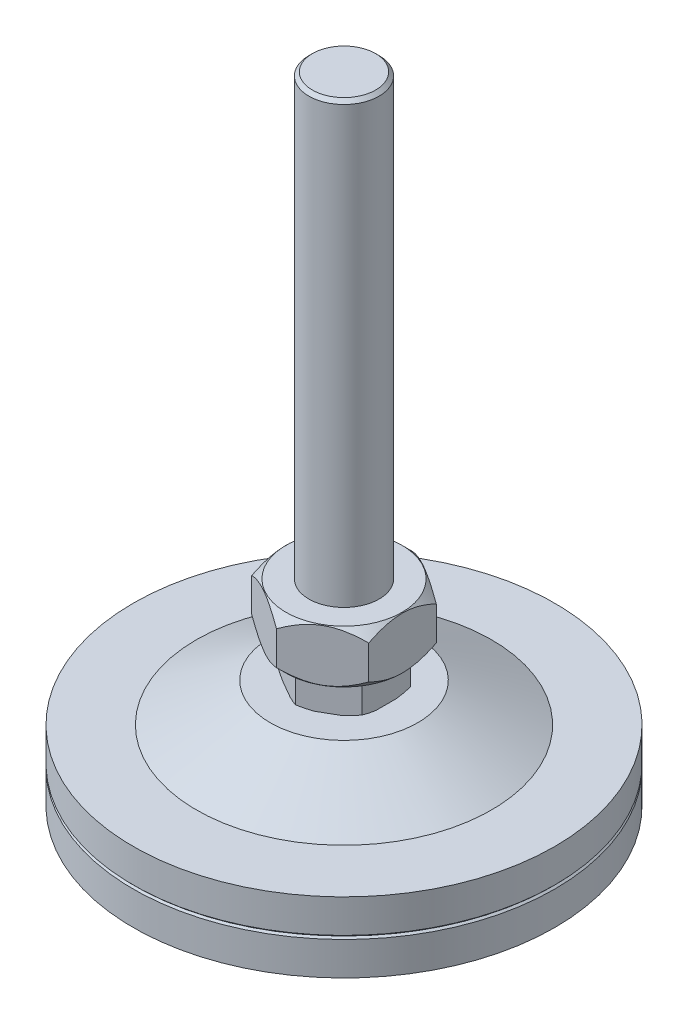
from build123d import *

# Parameters (mm, degrees)
BOSS_EXTRUDE1_DEPTH = 9
BOSS_EXTRUDE2_START = 15
SKETCH5_R           = 10
BOSS_EXTRUDE2_DEPTH = 15
CHAMFER1_SIZE       = 1


with BuildPart() as part:
    # Sketch1 → Revolve1 (revolve)
    with BuildSketch(Plane.XY, mode=Mode.PRIVATE) as revolve1_sk:
        Polygon((35, 0), (60, 0), (60, 9.5), (59.5, 10), (60, 10.5), (60, 20), (42, 20), (21, 31), (10, 31), (10, 181), (0, 181), (0, 15), (14, 15), align=None)
    revolve(revolve1_sk.sketch.rotate(Axis((0, 181, 0), (0, -1, 0)), 180), axis=Axis((0, 181, 0), (0, -1, 0)))

    # Sketch2 → Boss-Extrude1 (add)
    with BuildSketch(Plane(origin=(0, 31, 0), x_dir=(1, 0, 0), z_dir=(0, 1, 0))):
        Polygon((12, 6.92820323), (0, 13.856406461), (-12, 6.92820323), (-12, -6.92820323), (0, -13.856406461), (12, -6.92820323), align=None)
    extrude(amount=BOSS_EXTRUDE1_DEPTH)

    # Sketch3 → Cut-Revolve1 (revolve, cut)
    with BuildSketch(Plane(origin=(0, 0, 0), x_dir=(0, 0, -1), z_dir=(1, 0, 0))):
        Polygon((12.356406461, 31), (13.856406461, 31.866025404), (13.856406461, 31), align=None)
        Polygon((13.856406461, 39.422649731), (12.856406461, 40), (13.856406461, 40), align=None)
    revolve(axis=Axis((0, 181, 0), (0, 1, 0)), mode=Mode.SUBTRACT)

    # Sketch5 → Boss-Extrude2 (add)
    with BuildSketch(Plane(origin=(0, 41, 0), x_dir=(-1, 0, 0), z_dir=(0, 1, 0)).offset(BOSS_EXTRUDE2_START)):
        Polygon((0, 19.225763964), (-16.65, 9.612881982), (-16.65, -9.612881982), (0, -19.225763964), (16.65, -9.612881982), (16.65, 9.612881982), align=None)
        with Locations(Location((0, 0, 0), (0, 0, 90))):
            Circle(SKETCH5_R, mode=Mode.SUBTRACT)
    extrude(amount=-BOSS_EXTRUDE2_DEPTH)

    # Sketch7 → Cut-Revolve3 (revolve, cut)
    with BuildSketch(Plane(origin=(0, 0, 0), x_dir=(0, 0, -1), z_dir=(1, 0, 0)), mode=Mode.PRIVATE) as cut_revolve3_sk:
        Polygon((16.525763964, 56), (19.225763964, 53.3), (19.225763964, 56), align=None)
        Polygon((16.525763964, 41), (19.225763964, 43.7), (19.225763964, 41), align=None)
    revolve(cut_revolve3_sk.sketch.rotate(Axis((0, 181, 0), (0, 1, 0)), 180), axis=Axis((0, 181, 0), (0, 1, 0)), mode=Mode.SUBTRACT)

    # Chamfer1
    chamfer1_edges = [part.edges().sort_by_distance(p)[0] for p in [
        (10, 181, 0),
    ]]
    chamfer(chamfer1_edges, length=CHAMFER1_SIZE)


solid = part.part
